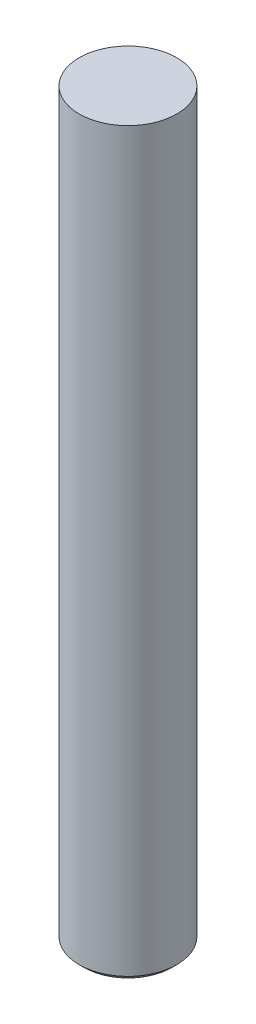
SolidWorks part; units mm, degrees
ref_plane "Front Plane" through (0, 0, 0) normal (0, 0, 1) x (1, 0, 0)
ref_plane "Top Plane" through (0, 0, 0) normal (0, 1, 0) x (1, 0, 0)
ref_plane "Right Plane" through (0, 0, 0) normal (1, 0, 0) x (0, 0, -1)
sketch "Sketch1" plane through (0, 0, 0) normal (0, 1, 0) x (1, 0, 0)
  circle A0 centre (0, 0) radius 10
  dimension "D1" = 20
extrude "Boss-Extrude1" add sketch "Sketch1" along normal mid plane 152
cosmetic thread "Cosmetic Thread1" parameters "D1"=40, "D2"=17.294
chamfer "Chamfer1" distance 1 angle 45 1 edges at (0, -76, 10)
ref_plane "Plane1" through (0, -36, 0) normal (0, -1, 0) x (-1, 0, 0)
